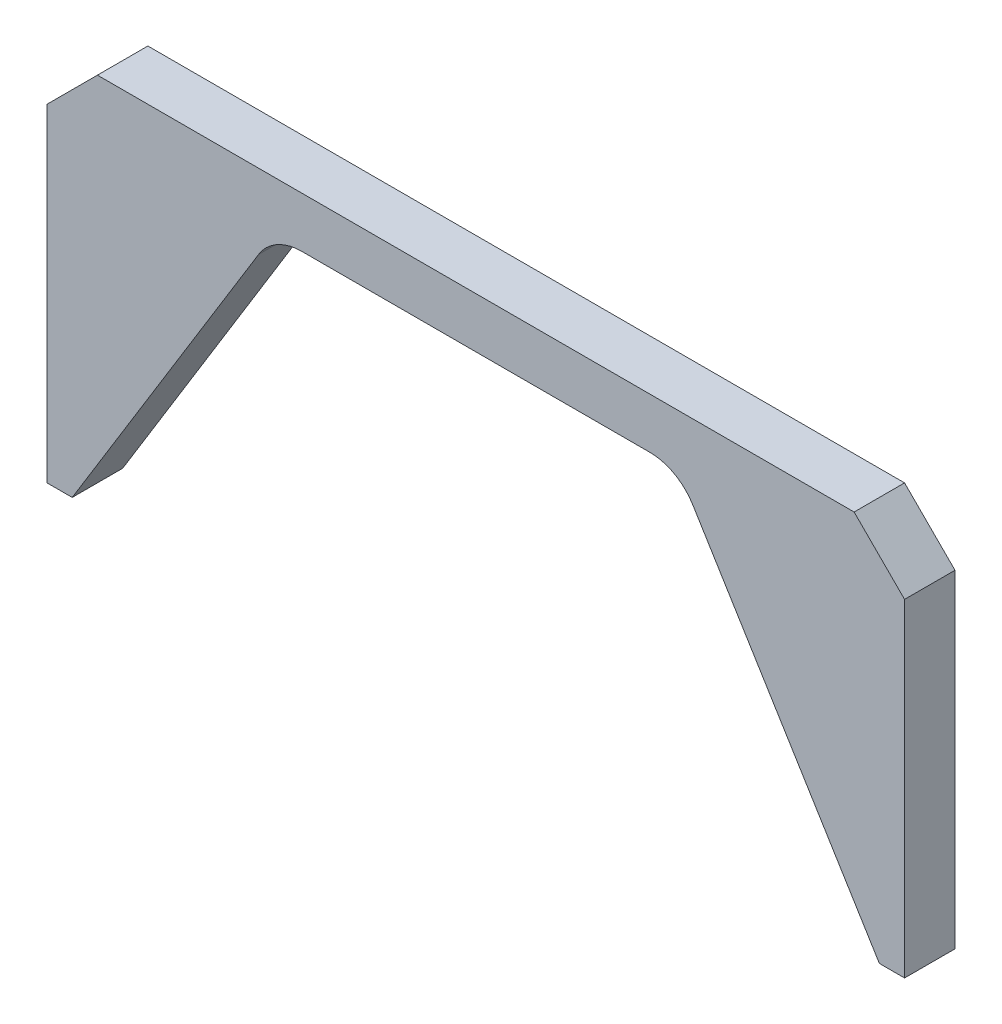
SolidWorks part; units mm, degrees
material "Q235B"
ref_plane "Front Plane" through (0, 0, 0) normal (0, 0, 1) x (1, 0, 0)
ref_plane "Top Plane" through (0, 0, 0) normal (0, 1, 0) x (1, 0, 0)
ref_plane "Right Plane" through (0, 0, 0) normal (1, 0, 0) x (0, 0, -1)
sketch "Sketch1" plane through (0, 0, 0) normal (0, 0, 1) x (1, 0, 0)
  line L0 (-85, 0) -> (-80, 0)
  line L1 (-80, 0) -> (-43.0221, 60.2319)
  line L2 (-34.5, 65) -> (34.5, 65)
  line L3 (0, 65) -> (0, 75) construction
  line L4 (85, 75) -> (-85, 75)
  line L5 (-85, 75) -> (-85, 0)
  line L6 (85, 75) -> (85, 0)
  line L7 (80, 0) -> (43.0221, 60.2319)
  line L8 (85, 0) -> (80, 0)
  arc A0 (43.0221, 60.2319) -> (34.5, 65) centre (34.5, 55) ccw
  arc A1 (-43.0221, 60.2319) -> (-34.5, 65) centre (-34.5, 55) cw
  point P13 (40.0949, 65)
  point P16 (-40.0949, 65)
  dimension "D5" = 10
  dimension "D1" = 170
  dimension "D2" = 160
  dimension "D3" = 65
  dimension "D4" = 75
  dimension "D6" = 69
extrude "Boss-Extrude1" add sketch "Sketch1" along normal mid plane 10
chamfer "Chamfer1" distance 10 angle 45 2 edges at (85, 75, 0) (-85, 75, 0)
